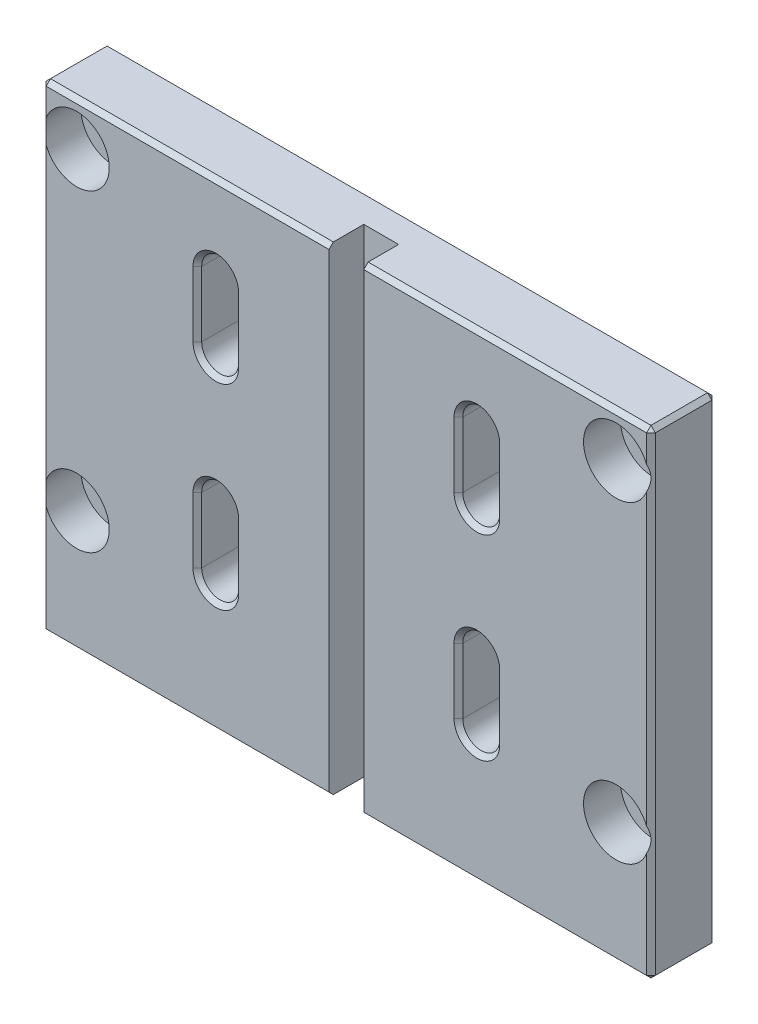
SolidWorks part; units mm, degrees
material "45#"
ref_plane "前视" through (0, 0, 0) normal (0, 0, 1) x (1, 0, 0)
ref_plane "上视" through (0, 0, 0) normal (0, 1, 0) x (1, 0, 0)
ref_plane "右视" through (0, 0, 0) normal (1, 0, 0) x (0, 0, -1)
sketch "草图1" plane through (0, 0, 0) normal (0, 0, 1) x (1, 0, 0)
  line L1 (70, -55) -> (-70, -55)
  line L2 (70, -55) -> (70, 55)
  line L3 (70, 55) -> (-70, 55)
  line L4 (-70, -55) -> (-70, 55)
  line L5 (70, -55) -> (-70, 55) construction
  line L6 (70, 55) -> (-70, -55) construction
  point P0 (0, 0)
  dimension "D1" = 140
  dimension "D2" = 110
extrude "凸台-拉伸1" add sketch "草图1" along normal mid plane 15
chamfer "倒角1" [suppressed] distance 0.5 angle 45
sketch "草图4" plane through (0, 0, -7.5) normal (0, 0, -1) x (-1, 0, 0)
  line L0 (-30, -10) -> (-30, -25) construction
  line L1 (-25.75, -10) -> (-25.75, -25)
  line L2 (-34.25, -10) -> (-34.25, -25)
  line L4 (-30, 35) -> (-30, 20) construction
  line L5 (-25.75, 35) -> (-25.75, 20)
  line L6 (-34.25, 35) -> (-34.25, 20)
  line L7 (0, 53.1664) -> (0, -72.5638) construction
  line L8 (30, 35) -> (30, 20) construction
  line L9 (25.75, 35) -> (25.75, 20)
  line L10 (34.25, 35) -> (34.25, 20)
  line L11 (30, -10) -> (30, -25) construction
  line L12 (25.75, -10) -> (25.75, -25)
  line L13 (34.25, -10) -> (34.25, -25)
  arc A0 (-25.75, -10) -> (-34.25, -10) centre (-30, -10) ccw
  arc A1 (-34.25, -25) -> (-25.75, -25) centre (-30, -25) ccw
  arc A2 (-25.75, 35) -> (-34.25, 35) centre (-30, 35) ccw
  arc A3 (-34.25, 20) -> (-25.75, 20) centre (-30, 20) ccw
  arc A4 (25.75, 35) -> (34.25, 35) centre (30, 35) cw
  arc A5 (34.25, 20) -> (25.75, 20) centre (30, 20) cw
  arc A6 (25.75, -10) -> (34.25, -10) centre (30, -10) cw
  arc A7 (34.25, -25) -> (25.75, -25) centre (30, -25) cw
  point P2 (-30, -17.5)
  point P10 (-30, 27.5)
  point P19 (30, 27.5)
  point P26 (30, -17.5)
  dimension "D1" = 4.25
  dimension "D2" = 15
  dimension "D3" = 30
  dimension "D4" = 10
  dimension "D5" = 45
extrude "切除-拉伸1" cut sketch "草图4" against normal through all contours A0 L2 A1 L1
chamfer "倒角2" distance 1 angle 45 44 edges at (25.75, -17.5, 7.5) (30, -29.25, 7.5) (34.25, -17.5, 7.5) (30, -5.75, 7.5) (-34.25, -17.5, 7.5) (-30, -29.25, 7.5) (-25.75, -17.5, 7.5) (-30, -5.75, 7.5) (-34.25, 27.5, 7.5) (-30, 15.75, 7.5) (-25.75, 27.5, 7.5) (-30, 39.25, 7.5) (25.75, 27.5, 7.5) (30, 15.75, 7.5) (34.25, 27.5, 7.5) (30, 39.25, 7.5) (-70, 55, 0) (70, 55, 0) (-70, -55, 0) (0, 55, 7.5) (70, 0, 7.5) (-70, 0, 7.5) (0, -55, 7.5) (70, -55, 0) (0, -55, -7.5) (70, 0, -7.5) (0, 55, -7.5) (-70, 0, -7.5) (30, -29.25, -7.5) (25.75, -17.5, -7.5) (30, -5.75, -7.5) (34.25, -17.5, -7.5) (-30, -29.25, -7.5) (-34.25, -17.5, -7.5) (-30, -5.75, -7.5) (-25.75, -17.5, -7.5) (-30, 15.75, -7.5) (-34.25, 27.5, -7.5) (-30, 39.25, -7.5) (-25.75, 27.5, -7.5) (30, 15.75, -7.5) (25.75, 27.5, -7.5) (30, 39.25, -7.5) (34.25, 27.5, -7.5)
sketch "草图5" plane through (0, 55, 0) normal (0, 1, 0) x (1, 0, 0)
  line L1 (-4, -15.5) -> (4, -15.5)
  line L2 (-4, -15.5) -> (-4, 0.5)
  line L3 (-4, 0.5) -> (4, 0.5)
  line L4 (4, -15.5) -> (4, 0.5)
  line L5 (-4, -15.5) -> (4, 0.5) construction
  line L6 (-4, 0.5) -> (4, -15.5) construction
  point P0 (0, -7.5)
  dimension "D1" = 8
  dimension "D2" = 16
extrude "切除-拉伸2" cut sketch "草图5" against normal through all
hole_wizard "M5 螺纹孔1" positions "草图6" profile "草图8" tap size "M5" standard "AS" end condition through all
sketch "草图6" plane through (0, 0, -7.5) normal (0, 0, -1) x (-1, 0, 0)
  line L0 (-69, 55) -> (69, 55) construction
  line L1 (-70, -54) -> (-70, 54) construction
  line L2 (70, 54) -> (70, -54) construction
  point P0 (-62, 45)
  point P2 (-62, -27)
  point P4 (62, -27)
  point P6 (62, 45)
  dimension "D1" = 10
  dimension "D2" = 8
  dimension "D3" = 8
sketch "草图8" plane through (62, 45, -7.5) normal (1, 0, 0) x (0, 1, 0)
  line L0 (0, 0) -> (0, 15)
  line L1 (0, 15) -> (2.1, 15)
  line L2 (2.1, 15) -> (2.1, 0)
  line L5 (2.1, 0) -> (0, 0)
  line L11 (0, -6.35) -> (0, 107.95) construction
  dimension "通孔螺纹孔钻头直径" = 4.2
  dimension "通孔螺纹孔钻头深度" = 15
cosmetic thread "孔螺蚊线1" parameters "D2"=5
cosmetic thread "孔螺蚊线2" parameters "D2"=5
cosmetic thread "孔螺蚊线3" parameters "D2"=5
cosmetic thread "孔螺蚊线4" parameters "D2"=5
hole_wizard "M5 螺纹孔2" positions "草图9" profile "草图10" tap size "M5" standard "GB"
sketch "草图9" plane through (0, -55, 0) normal (0, -1, 0) x (-1, 0, 0)
  point P0 (45, 0)
  point P2 (-45, 0)
  dimension "D1" = 45
  dimension "D2" = 45
sketch "草图10" plane through (-45, -55, 0) normal (1, 0, 0) x (0, 0, -1)
  line L0 (0, 0) -> (0, 13.6618)
  line L1 (0, 13.6618) -> (2.1, 12.4)
  line L2 (2.1, 12.4) -> (2.1, 0.425)
  line L3 (2.1, 0.425) -> (2.525, 0)
  line L5 (2.525, 0) -> (0, 0)
  line L6 (-2.1, 0.425) -> (-2.525, 0) construction
  line L10 (0, 13.6618) -> (-2.1, 12.4) construction
  line L11 (0, -6.35) -> (0, 107.95) construction
  dimension "螺纹孔钻头直径" = 4.2
  dimension "螺纹孔钻头深度" = 12.4
  dimension "近端锥形沉头孔直径" = 5.05
  dimension "近端锥形沉头孔角度" = 90
  dimension "导头角度" = 118
cosmetic thread "孔螺蚊线5" parameters "D1"=10, "D2"=5
cosmetic thread "孔螺蚊线6" parameters "D1"=10, "D2"=5
hole_wizard "Hole1" positions "Point_Sketch" profile "Profil_Sketch" counterbore size "M6" standard "ISO" end condition through all
sketch "Point_Sketch" plane through (49.1309, -26.065, 7.5) normal (0, 0, -1) x (1, 0, 0)
  line L0 (-49.1309, 27.935) -> (-49.1309, -39.1534) construction
  line L1 (19.8691, 27.935) -> (-118.1309, 27.935) construction
  point P0 (12.8691, 0.935)
  point P2 (12.8691, -71.065)
  point P12 (-111.1309, -71.065)
  point P13 (-111.1309, 0.935)
sketch "Profil_Sketch" plane through (62, -27, 7.5) normal (1, 0, 0) x (0, -1, 0)
  line L0 (0, 0) -> (0, 15)
  line L1 (0, 15) -> (4.5, 15)
  line L3 (4.5, 15) -> (4.5, 8.5)
  line L4 (4.5, 8.5) -> (7.5, 8.5)
  line L5 (7.5, 8.5) -> (7.5, 0)
  line L7 (7.5, 0) -> (0, 0)
  line L11 (0, -6.35) -> (0, 107.95) construction
  dimension "Diameter" = 9
  dimension "Thru Hole Depth" = 15
  dimension "L1" = 8.5
other "usin_LS160_M8x22-SH<1>"
